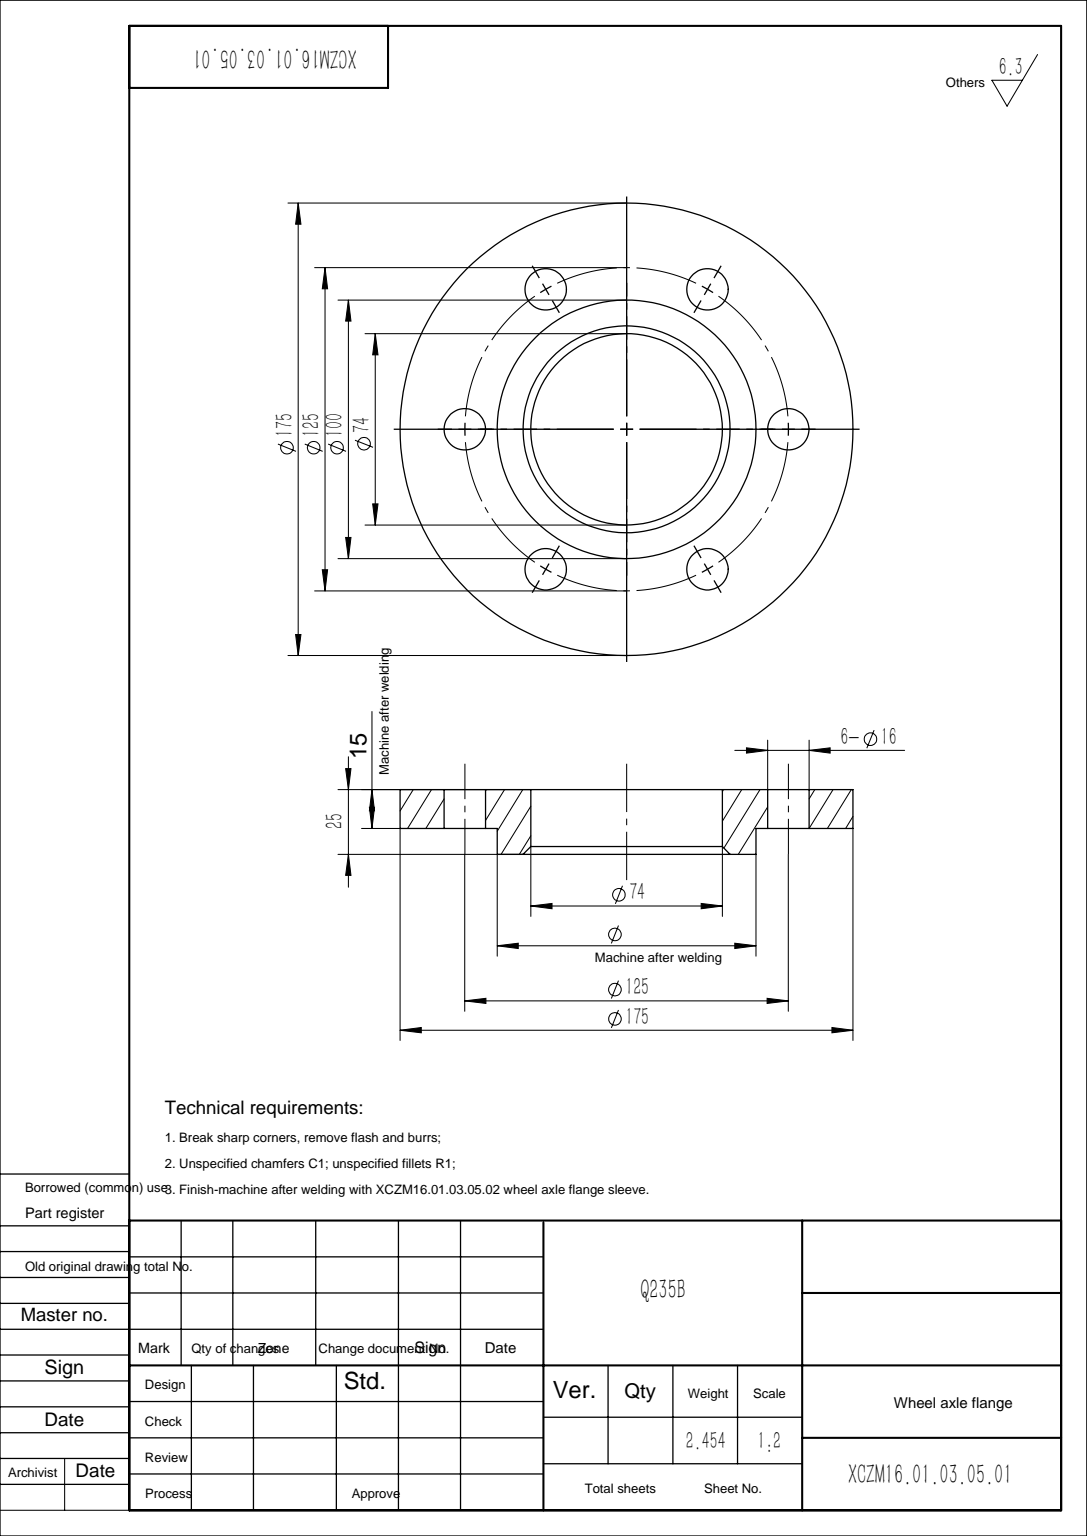
from build123d import *

# Parameters (mm, degrees)
SKETCH1_R                  = 50
BOSS_EXTRUDE1_DEPTH        = 10
SKETCH2_R                  = 87.5
BOSS_EXTRUDE2_DEPTH        = 15
CUT_EXTRUDE1_REACH         = 128.244
SKETCH3_R                  = 37
F_16_0_16_DIAMETER_HOLE1_D = 16
CHAMFER1_SIZE              = 3


with BuildPart() as part:
    # Sketch1 → Boss-Extrude1 (new body)
    with BuildSketch(Plane.XY):
        Circle(SKETCH1_R)
    extrude(amount=BOSS_EXTRUDE1_DEPTH)

    # Sketch2 → Boss-Extrude2 (add)
    with BuildSketch(Plane.XY):
        Circle(SKETCH2_R)
    extrude(amount=-BOSS_EXTRUDE2_DEPTH)

    # Sketch3 → Cut-Extrude1 (cut, up to next)
    with BuildSketch(Plane.XY.offset(10), mode=Mode.PRIVATE) as cut_extrude1_sk1:
        Circle(SKETCH3_R)
    cut_extrude1_tool1 = extrude(cut_extrude1_sk1.sketch, amount=-CUT_EXTRUDE1_REACH, mode=Mode.PRIVATE) & part.part
    add(cut_extrude1_tool1.solids().sort_by_distance((0, 0, 10))[0], mode=Mode.SUBTRACT)

    # Ø16.0 (16) Diameter Hole1 (through all)
    with Locations(Plane.XY):
        with Locations((62.5, 0), (31.25, -54.126587737), (-31.25, -54.126587737), (-62.5, 0), (-31.25, 54.126587737), (31.25, 54.126587737)):
            Hole(F_16_0_16_DIAMETER_HOLE1_D / 2)

    # Chamfer1
    chamfer1_edges = [part.edges().sort_by_distance(p)[0] for p in [
        (-37, 0, 10),
    ]]
    chamfer(chamfer1_edges, length=CHAMFER1_SIZE)


solid = part.part
